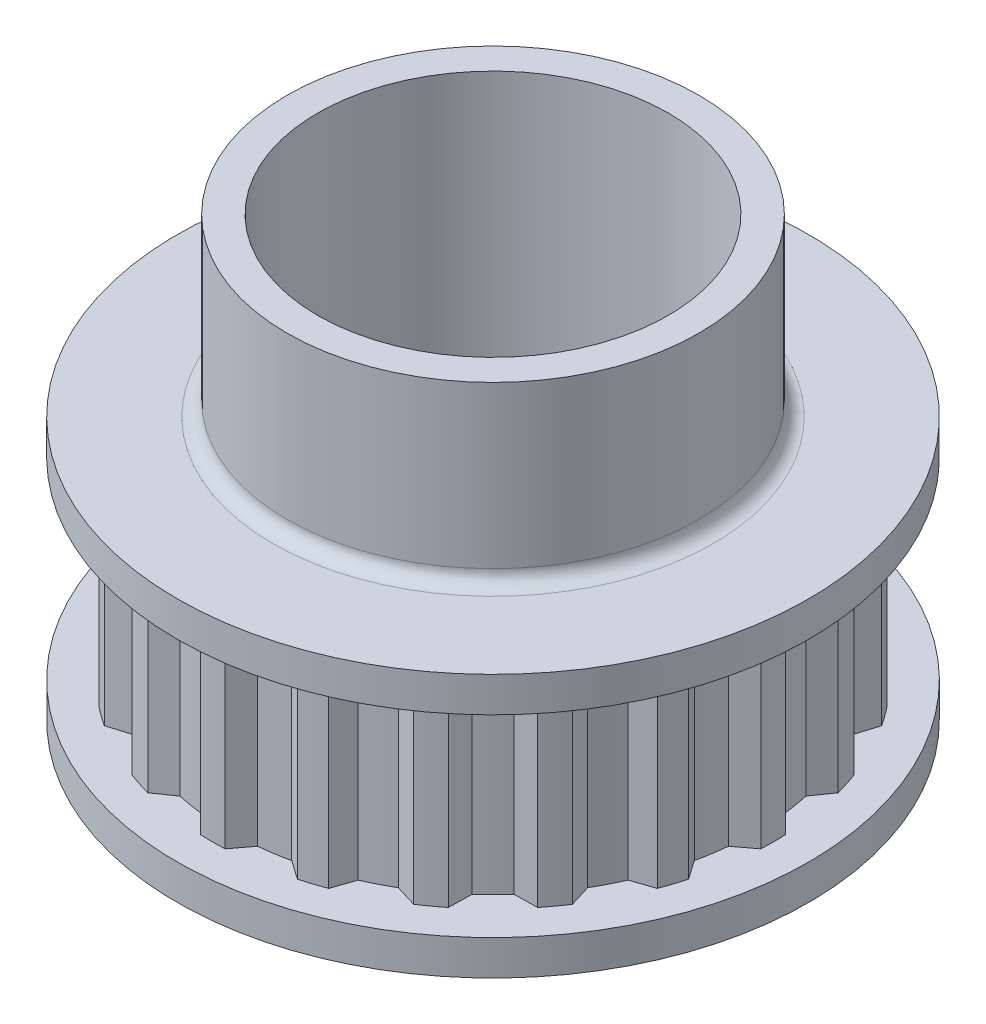
from build123d import *

# Parameters (mm, degrees)
SKETCH1_R           = 16
BOSS_EXTRUDE1_DEPTH = 11
CUT_EXTRUDE2_START  = -21
CUT_EXTRUDE2_DEPTH  = 21
SKETCH3_R           = 18
BOSS_EXTRUDE2_DEPTH = 2
BOSS_EXTRUDE3_START = 2
SKETCH4_R           = 18
BOSS_EXTRUDE3_DEPTH = 2
SKETCH5_R           = 11.75
BOSS_EXTRUDE4_DEPTH = 10
FILLET1_R           = 0.8
SKETCH6_R           = 10
CUT_EXTRUDE3_DEPTH  = 51


with BuildPart() as part:
    # Sketch1 → Boss-Extrude1 (new body)
    with BuildSketch(Plane(origin=(0, 0, 0), x_dir=(1, 0, 0), z_dir=(0, 1, 0))):
        with Locations(Location((0, 0, 0), (0, 0, 270))):
            Circle(SKETCH1_R)
    extrude(amount=BOSS_EXTRUDE1_DEPTH)

    # Sketch2 → Cut-Extrude2 (cut)
    with BuildSketch(Plane(origin=(0, 11, 0), x_dir=(1, 0, 0), z_dir=(0, 1, 0)).offset(CUT_EXTRUDE2_START)):
        with BuildLine():
            ThreePointArc((4.265167024, 15.421035966), (2.502951441, 15.80301345), (0.708947293, 15.984285838))
            Line((0.708947293, 15.984285838), (1.5, 14.932939883))
            ThreePointArc((1.5, 14.932939883), (2.347782156, 14.823313142), (3.187947426, 14.665595275))
            Line((3.187947426, 14.665595275), (4.265167024, 15.421035966))
        make_face()
        with BuildLine():
            ThreePointArc((8.821777076, 13.348267649), (7.263847996, 14.256104387), (5.613664909, 14.982882443))
            Line((5.613664909, 14.982882443), (6.041116974, 13.738544292))
            ThreePointArc((6.041116974, 13.738544292), (6.813529192, 13.372303972), (7.563836345, 12.96268002))
            Line((7.563836345, 12.96268002), (8.821777076, 13.348267649))
        make_face()
        with BuildLine():
            ThreePointArc((12.514850122, 9.968877892), (11.313708499, 11.313708499), (9.968877892, 12.514850122))
            Line((9.968877892, 12.514850122), (9.990887328, 11.199324263))
            ThreePointArc((9.990887328, 11.199324263), (10.612320518, 10.612320518), (11.199324263, 9.990887328))
            Line((11.199324263, 9.990887328), (12.514850122, 9.968877892))
        make_face()
        with BuildLine():
            ThreePointArc((14.982882443, 5.613664909), (14.256104387, 7.263847996), (13.348267649, 8.821777076))
            Line((13.348267649, 8.821777076), (12.96268002, 7.563836345))
            ThreePointArc((12.96268002, 7.563836345), (13.372303972, 6.813529192), (13.738544292, 6.041116974))
            Line((13.738544292, 6.041116974), (14.982882443, 5.613664909))
        make_face()
        with BuildLine():
            ThreePointArc((15.984285838, 0.708947293), (15.80301345, 2.502951441), (15.421035966, 4.265167024))
            Line((15.421035966, 4.265167024), (14.665595275, 3.187947426))
            ThreePointArc((14.665595275, 3.187947426), (14.823313142, 2.347782156), (14.932939883, 1.5))
            Line((14.932939883, 1.5), (15.984285838, 0.708947293))
        make_face()
        with BuildLine():
            ThreePointArc((15.421035966, -4.265167024), (15.80301345, -2.502951441), (15.984285838, -0.708947293))
            Line((15.984285838, -0.708947293), (14.932939883, -1.5))
            ThreePointArc((14.932939883, -1.5), (14.823313142, -2.347782156), (14.665595275, -3.187947426))
            Line((14.665595275, -3.187947426), (15.421035966, -4.265167024))
        make_face()
        with BuildLine():
            ThreePointArc((13.348267649, -8.821777076), (14.256104387, -7.263847996), (14.982882443, -5.613664909))
            Line((14.982882443, -5.613664909), (13.738544292, -6.041116974))
            ThreePointArc((13.738544292, -6.041116974), (13.372303972, -6.813529192), (12.96268002, -7.563836345))
            Line((12.96268002, -7.563836345), (13.348267649, -8.821777076))
        make_face()
        with BuildLine():
            ThreePointArc((9.968877892, -12.514850122), (11.313708499, -11.313708499), (12.514850122, -9.968877892))
            Line((12.514850122, -9.968877892), (11.199324263, -9.990887328))
            ThreePointArc((11.199324263, -9.990887328), (10.612320518, -10.612320518), (9.990887328, -11.199324263))
            Line((9.990887328, -11.199324263), (9.968877892, -12.514850122))
        make_face()
        with BuildLine():
            ThreePointArc((5.613664909, -14.982882443), (7.263847996, -14.256104387), (8.821777076, -13.348267649))
            Line((8.821777076, -13.348267649), (7.563836345, -12.96268002))
            ThreePointArc((7.563836345, -12.96268002), (6.813529192, -13.372303972), (6.041116974, -13.738544292))
            Line((6.041116974, -13.738544292), (5.613664909, -14.982882443))
        make_face()
        with BuildLine():
            Line((1.5, -14.932939883), (0.708947293, -15.984285838))
            ThreePointArc((0.708947293, -15.984285838), (2.502951441, -15.80301345), (4.265167024, -15.421035966))
            Line((4.265167024, -15.421035966), (3.187947426, -14.665595275))
            ThreePointArc((3.187947426, -14.665595275), (2.347782156, -14.823313142), (1.5, -14.932939883))
        make_face()
        with BuildLine():
            Line((-3.187947426, -14.665595275), (-4.265167024, -15.421035966))
            ThreePointArc((-4.265167024, -15.421035966), (-2.502951441, -15.80301345), (-0.708947293, -15.984285838))
            Line((-0.708947293, -15.984285838), (-1.5, -14.932939883))
            ThreePointArc((-1.5, -14.932939883), (-2.347782156, -14.823313142), (-3.187947426, -14.665595275))
        make_face()
        with BuildLine():
            Line((-7.563836345, -12.96268002), (-8.821777076, -13.348267649))
            ThreePointArc((-8.821777076, -13.348267649), (-7.263847996, -14.256104387), (-5.613664909, -14.982882443))
            Line((-5.613664909, -14.982882443), (-6.041116974, -13.738544292))
            ThreePointArc((-6.041116974, -13.738544292), (-6.813529192, -13.372303972), (-7.563836345, -12.96268002))
        make_face()
        with BuildLine():
            Line((-11.199324263, -9.990887328), (-12.514850122, -9.968877892))
            ThreePointArc((-12.514850122, -9.968877892), (-11.313708499, -11.313708499), (-9.968877892, -12.514850122))
            Line((-9.968877892, -12.514850122), (-9.990887328, -11.199324263))
            ThreePointArc((-9.990887328, -11.199324263), (-10.612320518, -10.612320518), (-11.199324263, -9.990887328))
        make_face()
        with BuildLine():
            Line((-13.738544292, -6.041116974), (-14.982882443, -5.613664909))
            ThreePointArc((-14.982882443, -5.613664909), (-14.256104387, -7.263847996), (-13.348267649, -8.821777076))
            Line((-13.348267649, -8.821777076), (-12.96268002, -7.563836345))
            ThreePointArc((-12.96268002, -7.563836345), (-13.372303972, -6.813529192), (-13.738544292, -6.041116974))
        make_face()
        with BuildLine():
            Line((-14.932939883, -1.5), (-15.984285838, -0.708947293))
            ThreePointArc((-15.984285838, -0.708947293), (-15.80301345, -2.502951441), (-15.421035966, -4.265167024))
            Line((-15.421035966, -4.265167024), (-14.665595275, -3.187947426))
            ThreePointArc((-14.665595275, -3.187947426), (-14.823313142, -2.347782156), (-14.932939883, -1.5))
        make_face()
        with BuildLine():
            Line((-14.665595275, 3.187947426), (-15.421035966, 4.265167024))
            ThreePointArc((-15.421035966, 4.265167024), (-15.80301345, 2.502951441), (-15.984285838, 0.708947293))
            Line((-15.984285838, 0.708947293), (-14.932939883, 1.5))
            ThreePointArc((-14.932939883, 1.5), (-14.823313142, 2.347782156), (-14.665595275, 3.187947426))
        make_face()
        with BuildLine():
            Line((-12.96268002, 7.563836345), (-13.348267649, 8.821777076))
            ThreePointArc((-13.348267649, 8.821777076), (-14.256104387, 7.263847996), (-14.982882443, 5.613664909))
            Line((-14.982882443, 5.613664909), (-13.738544292, 6.041116974))
            ThreePointArc((-13.738544292, 6.041116974), (-13.372303972, 6.813529192), (-12.96268002, 7.563836345))
        make_face()
        with BuildLine():
            Line((-9.990887328, 11.199324263), (-9.968877892, 12.514850122))
            ThreePointArc((-9.968877892, 12.514850122), (-11.313708499, 11.313708499), (-12.514850122, 9.968877892))
            Line((-12.514850122, 9.968877892), (-11.199324263, 9.990887328))
            ThreePointArc((-11.199324263, 9.990887328), (-10.612320518, 10.612320518), (-9.990887328, 11.199324263))
        make_face()
        with BuildLine():
            Line((-6.041116974, 13.738544292), (-5.613664909, 14.982882443))
            ThreePointArc((-5.613664909, 14.982882443), (-7.263847996, 14.256104387), (-8.821777076, 13.348267649))
            Line((-8.821777076, 13.348267649), (-7.563836345, 12.96268002))
            ThreePointArc((-7.563836345, 12.96268002), (-6.813529192, 13.372303972), (-6.041116974, 13.738544292))
        make_face()
        with BuildLine():
            ThreePointArc((-3.187947426, 14.665595275), (-2.347782156, 14.823313142), (-1.5, 14.932939883))
            Line((-1.5, 14.932939883), (-0.708947293, 15.984285838))
            ThreePointArc((-0.708947293, 15.984285838), (-2.502951441, 15.80301345), (-4.265167024, 15.421035966))
            Line((-4.265167024, 15.421035966), (-3.187947426, 14.665595275))
        make_face()
    extrude(amount=CUT_EXTRUDE2_DEPTH, mode=Mode.SUBTRACT)

    # Sketch3 → Boss-Extrude2 (add)
    with BuildSketch(Plane(origin=(0, 11, 0), x_dir=(1, 0, 0), z_dir=(0, 1, 0))):
        with Locations(Location((0, 0, 0), (0, 0, 270))):
            Circle(SKETCH3_R)
    extrude(amount=BOSS_EXTRUDE2_DEPTH)

    # Sketch4 → Boss-Extrude3 (add)
    with BuildSketch(Plane.XZ.offset(BOSS_EXTRUDE3_START)):
        with Locations(Location((0, 0, 0), (0, 0, 90))):
            Circle(SKETCH4_R)
    extrude(amount=-BOSS_EXTRUDE3_DEPTH)

    # Sketch5 → Boss-Extrude4 (add)
    with BuildSketch(Plane(origin=(0, 13, 0), x_dir=(1, 0, 0), z_dir=(0, 1, 0))):
        with Locations(Location((0, 0, 0), (0, 0, 270))):
            Circle(SKETCH5_R)
    extrude(amount=BOSS_EXTRUDE4_DEPTH)

    # Fillet1
    fillet1_edges = [part.edges().sort_by_distance(p)[0] for p in [
        (0, 13, -11.75),
    ]]
    fillet(fillet1_edges, radius=FILLET1_R)

    # Sketch6 → Cut-Extrude3 (cut)
    with BuildSketch(Plane(origin=(0, 23, 0), x_dir=(1, 0, 0), z_dir=(0, 1, 0))):
        with Locations(Location((0, 0, 0), (0, 0, 270))):
            Circle(SKETCH6_R)
    extrude(amount=-CUT_EXTRUDE3_DEPTH, mode=Mode.SUBTRACT)


solid = part.part
